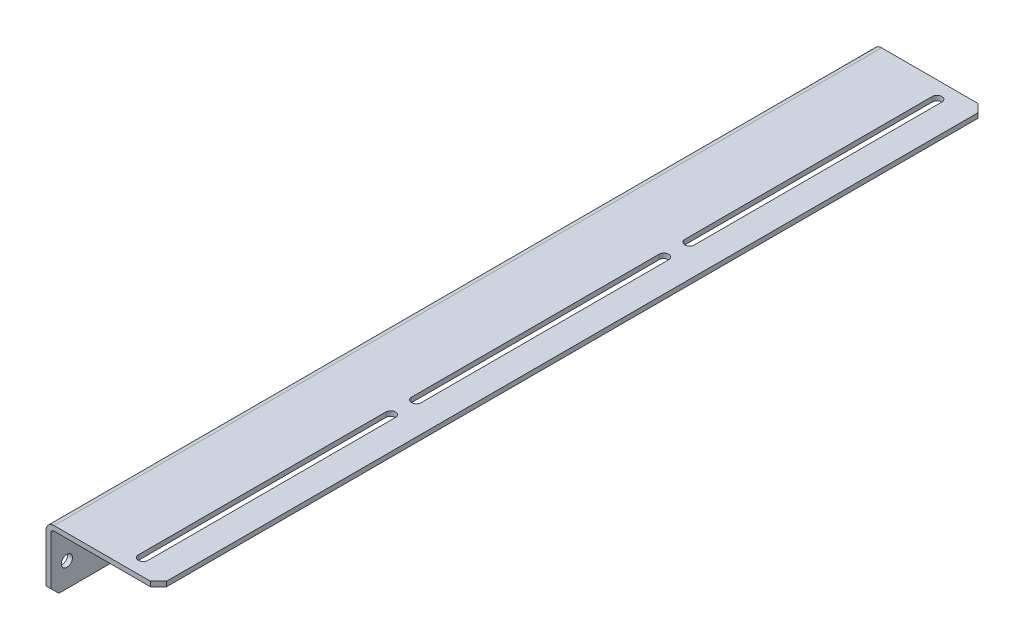
SolidWorks part; units mm, degrees
material "1023 碳钢板 (SS)"
ref_plane "前视基准面" through (0, 0, 0) normal (0, 0, 1) x (1, 0, 0)
ref_plane "上视基准面" through (0, 0, 0) normal (0, 1, 0) x (1, 0, 0)
ref_plane "右视基准面" through (0, 0, 0) normal (1, 0, 0) x (0, 0, -1)
sketch "草图1" plane through (0, 0, 0) normal (0, 0, 1) x (1, 0, 0)
  line L0 (0, 0) -> (-65, 0)
  line L1 (-70, -5) -> (-70, -40)
  line L2 (0, -3) -> (-65, -3)
  line L3 (-67, -5) -> (-67, -40)
  line L4 (0, 0) -> (0, -3)
  line L5 (-70, -40) -> (-67, -40)
  arc A0 (-65, 0) -> (-70, -5) centre (-65, -5) ccw
  arc A1 (-65, -3) -> (-67, -5) centre (-65, -5) ccw
  point P6 (-70, 0)
  dimension "D3" = 5
  dimension "D1" = 40
  dimension "D2" = 70
  dimension "D4" = 3
extrude "凸台-拉伸1" add sketch "草图1" along normal blind 515 contours L5 L3 A1 L2 L4 L0 A0 L1
sketch "草图3" plane through (-70, 0, 0) normal (-1, 0, 0) x (0, 0, 1)
  line L0 (0, -5) -> (0, -40) construction
  line L1 (515, 0) -> (0, 0) construction
  line L2 (257.5, -40) -> (257.5, -4.1506) construction
  line L3 (515, -40) -> (0, -40) construction
  circle A0 centre (10, -25) radius 3.5
  circle A1 centre (70, -25) radius 3.5
  circle A5 centre (287.5, -25) radius 3.5
  circle A6 centre (180, -25) radius 3.5
  circle A7 centre (120, -25) radius 3.5
  circle A9 centre (227.5, -25) radius 3.5
  circle A10 centre (445, -25) radius 3.5
  circle A11 centre (505, -25) radius 3.5
  circle A12 centre (395, -25) radius 3.5
  circle A13 centre (335, -25) radius 3.5
  dimension "D7" = 7
  dimension "D8" = 25
  dimension "D1" = 10
  dimension "D2" = 60
  dimension "D3" = 50
  dimension "D4" = 60
  dimension "D5" = 47.5
  dimension "D6" = 60
extrude "切除-拉伸1" cut sketch "草图3" against normal blind 515
chamfer "倒角1" distance 5 angle 45 4 edges at (0, -1.5, 515) (-68.5, -40, 515) (0, -1.5, 0) (-68.5, -40, 0)
sketch "草图4" plane through (0, 0, 0) normal (0, 1, 0) x (1, 0, 0)
  line L0 (-20, -10.5) -> (-20, -164.5) construction
  line L1 (-17, -10.5) -> (-17, -164.5)
  line L2 (-23, -10.5) -> (-23, -164.5)
  line L3 (0, -510) -> (0, -5) construction
  line L6 (-5, 0) -> (-65, 0) construction
  line L7 (-20, -180.5) -> (-20, -334.5) construction
  line L8 (-17, -180.5) -> (-17, -334.5)
  line L9 (-23, -180.5) -> (-23, -334.5)
  line L10 (-65, -257.5) -> (86.9042, -257.5) construction
  line L11 (-65, -515) -> (-65, 0) construction
  line L12 (-20, -504.5) -> (-20, -350.5) construction
  line L13 (-17, -504.5) -> (-17, -350.5)
  line L14 (-23, -504.5) -> (-23, -350.5)
  arc A0 (-17, -10.5) -> (-23, -10.5) centre (-20, -10.5) ccw
  arc A1 (-23, -164.5) -> (-17, -164.5) centre (-20, -164.5) ccw
  arc A2 (-17, -180.5) -> (-23, -180.5) centre (-20, -180.5) ccw
  arc A3 (-23, -334.5) -> (-17, -334.5) centre (-20, -334.5) ccw
  arc A4 (-17, -504.5) -> (-23, -504.5) centre (-20, -504.5) cw
  arc A5 (-23, -350.5) -> (-17, -350.5) centre (-20, -350.5) cw
  point P2 (-20, -87.5)
  point P13 (-20, -257.5)
  point P24 (-20, -427.5)
  dimension "D1" = 3
  dimension "D2" = 20
  dimension "D4" = 10.5
  dimension "D5" = 16
  dimension "D6" = 3
  dimension "D3" = 154
  dimension "D7" = 154
extrude "切除-拉伸2" cut sketch "草图4" against normal blind 515
